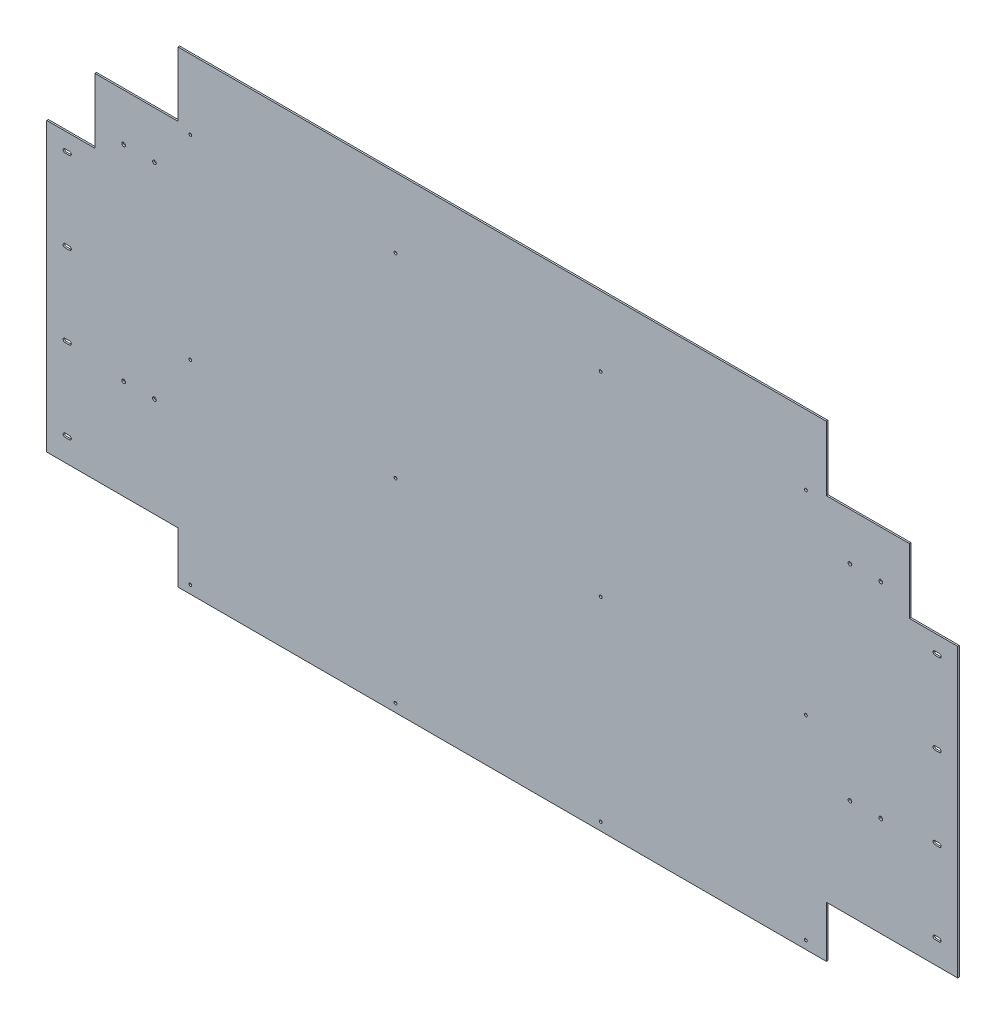
SolidWorks part; units mm, degrees
material "1023 碳钢板 (SS)"
ref_plane "Front Plane" through (0, 0, 0) normal (0, 0, 1) x (1, 0, 0)
ref_plane "Top Plane" through (0, 0, 0) normal (0, 1, 0) x (1, 0, 0)
ref_plane "Right Plane" through (0, 0, 0) normal (1, 0, 0) x (0, 0, -1)
sketch "Sketch1" plane through (0, 0, 0) normal (0, 0, 1) x (1, 0, 0)
  line L0 (-790, 570) -> (-790, 413)
  line L1 (-790, 570) -> (790, 570)
  line L2 (-1110, 255) -> (-1110, -445)
  line L3 (-790, -570) -> (790, -570)
  line L4 (1110, 255) -> (1110, -445)
  line L5 (-1110, 570) -> (1110, -570) construction
  line L6 (-1110, -570) -> (1110, 570) construction
  line L7 (-790, 413) -> (-992.5, 413)
  line L8 (-992.5, 413) -> (-992.5, 255)
  line L10 (-992.5, 255) -> (-1110, 255)
  line L11 (-1110, 255) -> (-1110, 570)
  line L12 (0, 570) -> (0, 0) construction
  line L13 (-1110, -445) -> (-790, -445)
  line L14 (-790, -445) -> (-790, -570)
  line L18 (790, -445) -> (790, -570)
  line L19 (1110, -445) -> (790, -445)
  line L22 (992.5, 255) -> (1110, 255)
  line L23 (992.5, 413) -> (992.5, 255)
  line L24 (790, 413) -> (992.5, 413)
  line L25 (790, 570) -> (790, 413)
  point P0 (0, 0)
  dimension "D1" = 2220
  dimension "D2" = 1140
  dimension "D3" = 320
  dimension "D4" = 202.5
  dimension "D5" = 158
  dimension "D6" = 157
  dimension "D7" = 320
  dimension "D8" = 125
extrude "Boss-Extrude1" add sketch "Sketch1" along normal blind 4 contours L10 L8 L7 L0 L1 L25 L24 L23 L22 L4 L19 L18 L3 L14 L13 L2
sketch "Sketch2" plane through (0, 0, 4) normal (0, 0, 1) x (1, 0, 0)
  line L0 (-1065.5, 213) -> (-1054.5, 213) construction
  line L1 (-1065.5, 217.5) -> (-1054.5, 217.5)
  line L2 (-1065.5, 208.5) -> (-1054.5, 208.5)
  line L3 (-1110, 255) -> (-1110, -445) construction
  line L4 (-992.5, 255) -> (-1110, 255) construction
  line L5 (-1065.5, 13) -> (-1054.5, 13) construction
  line L6 (-1065.5, 17.5) -> (-1054.5, 17.5)
  line L7 (-1065.5, 8.5) -> (-1054.5, 8.5)
  line L8 (-1065.5, -187) -> (-1054.5, -187) construction
  line L9 (-1065.5, -182.5) -> (-1054.5, -182.5)
  line L10 (-1065.5, -191.5) -> (-1054.5, -191.5)
  line L11 (-1065.5, -387) -> (-1054.5, -387) construction
  line L12 (-1065.5, -382.5) -> (-1054.5, -382.5)
  line L13 (-1065.5, -391.5) -> (-1054.5, -391.5)
  line L14 (0, 0) -> (0, 208.5) construction
  line L15 (1065.5, -387) -> (1054.5, -387) construction
  line L16 (1065.5, -382.5) -> (1054.5, -382.5)
  line L17 (1065.5, -391.5) -> (1054.5, -391.5)
  line L18 (1065.5, -187) -> (1054.5, -187) construction
  line L19 (1065.5, -182.5) -> (1054.5, -182.5)
  line L20 (1065.5, -191.5) -> (1054.5, -191.5)
  line L21 (1065.5, 13) -> (1054.5, 13) construction
  line L22 (1065.5, 17.5) -> (1054.5, 17.5)
  line L23 (1065.5, 8.5) -> (1054.5, 8.5)
  line L24 (1065.5, 213) -> (1054.5, 213) construction
  line L25 (1065.5, 217.5) -> (1054.5, 217.5)
  line L26 (1065.5, 208.5) -> (1054.5, 208.5)
  line L27 (-260, 400) -> (-260, -550) construction
  line L28 (-760, -550) -> (740, -550) construction
  line L29 (-760, -550) -> (-760, 400) construction
  line L30 (-760, 400) -> (740, 400) construction
  line L31 (740, -550) -> (740, 400) construction
  line L32 (-760, -550) -> (740, 400) construction
  line L33 (-760, 400) -> (740, -550) construction
  line L34 (-760, -75) -> (740, -75) construction
  line L35 (240, 400) -> (240, -550) construction
  line L36 (-790, 413) -> (-992.5, 413) construction
  line L37 (-922.5, 298) -> (-847.5, 298) construction
  line L38 (-922.5, 298) -> (-922.5, -202) construction
  line L39 (-922.5, -202) -> (-847.5, -202) construction
  line L40 (-847.5, 298) -> (-847.5, -202) construction
  line L41 (-922.5, 298) -> (-847.5, -202) construction
  line L42 (-922.5, -202) -> (-847.5, 298) construction
  line L43 (-992.5, 413) -> (-992.5, 255) construction
  line L44 (922.5, -202) -> (847.5, -202) construction
  line L45 (847.5, 298) -> (847.5, -202) construction
  line L46 (922.5, 298) -> (847.5, 298) construction
  line L47 (922.5, 298) -> (922.5, -202) construction
  line L48 (-790, -570) -> (790, -570) construction
  line L49 (1110, 255) -> (1110, -445) construction
  line L50 (-790, -445) -> (-790, -570) construction
  arc A0 (-1065.5, 217.5) -> (-1065.5, 208.5) centre (-1065.5, 213) ccw
  arc A1 (-1054.5, 208.5) -> (-1054.5, 217.5) centre (-1054.5, 213) ccw
  arc A2 (-1065.5, 17.5) -> (-1065.5, 8.5) centre (-1065.5, 13) ccw
  arc A3 (-1054.5, 8.5) -> (-1054.5, 17.5) centre (-1054.5, 13) ccw
  arc A4 (-1065.5, -182.5) -> (-1065.5, -191.5) centre (-1065.5, -187) ccw
  arc A5 (-1054.5, -191.5) -> (-1054.5, -182.5) centre (-1054.5, -187) ccw
  arc A6 (-1065.5, -382.5) -> (-1065.5, -391.5) centre (-1065.5, -387) ccw
  arc A7 (-1054.5, -391.5) -> (-1054.5, -382.5) centre (-1054.5, -387) ccw
  arc A8 (1065.5, -382.5) -> (1065.5, -391.5) centre (1065.5, -387) cw
  arc A9 (1054.5, -391.5) -> (1054.5, -382.5) centre (1054.5, -387) cw
  arc A10 (1065.5, -182.5) -> (1065.5, -191.5) centre (1065.5, -187) cw
  arc A11 (1054.5, -191.5) -> (1054.5, -182.5) centre (1054.5, -187) cw
  arc A12 (1065.5, 17.5) -> (1065.5, 8.5) centre (1065.5, 13) cw
  arc A13 (1054.5, 8.5) -> (1054.5, 17.5) centre (1054.5, 13) cw
  arc A14 (1065.5, 217.5) -> (1065.5, 208.5) centre (1065.5, 213) cw
  arc A15 (1054.5, 208.5) -> (1054.5, 217.5) centre (1054.5, 213) cw
  circle A16 centre (-760, 400) radius 3.5
  circle A17 centre (-260, 400) radius 3.5
  circle A18 centre (240, 400) radius 3.5
  circle A19 centre (740, 400) radius 3.5
  circle A20 centre (-760, -75) radius 3.5
  circle A21 centre (-260, -75) radius 3.5
  circle A22 centre (240, -75) radius 3.5
  circle A23 centre (740, -75) radius 3.5
  circle A24 centre (-760, -550) radius 3.5
  circle A25 centre (-260, -550) radius 3.5
  circle A26 centre (240, -550) radius 3.5
  circle A27 centre (740, -550) radius 3.5
  circle A28 centre (-922.5, 298) radius 4.5
  circle A29 centre (-847.5, 298) radius 4.5
  circle A30 centre (-922.5, -202) radius 4.5
  circle A31 centre (-847.5, -202) radius 4.5
  circle A32 centre (847.5, 298) radius 4.5
  circle A33 centre (922.5, 298) radius 4.5
  circle A34 centre (847.5, -202) radius 4.5
  circle A35 centre (922.5, -202) radius 4.5
  point P2 (-1060, 213)
  point P15 (-1060, 13)
  point P22 (-1060, -187)
  point P29 (-1060, -387)
  point P37 (1060, -387)
  point P44 (1060, -187)
  point P51 (1060, 13)
  point P58 (1060, 213)
  point P87 (-885, 48)
  dimension "D1" = 4.5
  dimension "D4" = 42
  dimension "D11" = 7
  dimension "D16" = 9
  dimension "D2" = 11
  dimension "D3" = 44.5
  dimension "D6" = 1500
  dimension "D7" = 950
  dimension "D8" = 500
  dimension "D9" = 475
  dimension "D10" = 500
  dimension "D12" = 500
  dimension "D13" = 115
  dimension "D14" = 70
  dimension "D15" = 75
  dimension "D17" = 20
  dimension "D18" = 44.5
  dimension "D19" = 30
  dimension "D5" = 4
extrude "Cut-Extrude1" cut sketch "Sketch2" against normal blind 4
